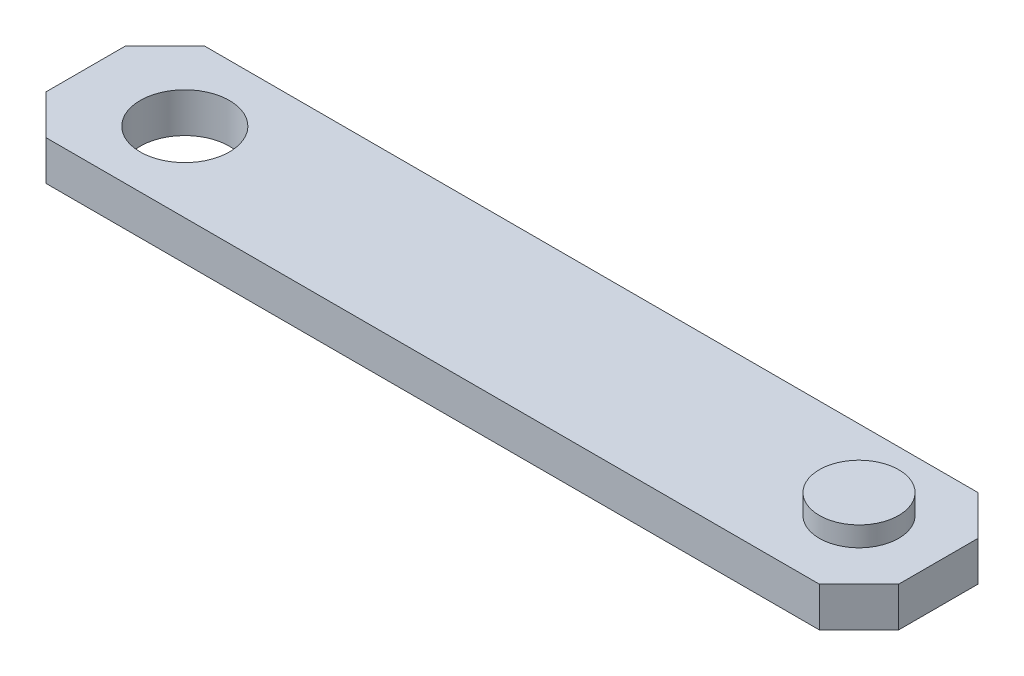
from build123d import *

# Parameters (mm, degrees)
SKETCH1_W           = 43
SKETCH1_H           = 8
BOSS_EXTRUDE1_DEPTH = 2
SKETCH2_R           = 2.25
CUT_EXTRUDE1_DEPTH  = 35.195745727
SKETCH3_R           = 2
BOSS_EXTRUDE2_DEPTH = 1
CHAMFER2_SIZE       = 2


with BuildPart() as part:
    # Sketch1 → Boss-Extrude1 (new body)
    with BuildSketch(Plane(origin=(0, 0, 0), x_dir=(1, 0, 0), z_dir=(0, 1, 0))):
        with Locations((11.806648575, 3.484396201)):
            Rectangle(SKETCH1_W, SKETCH1_H)
    extrude(amount=BOSS_EXTRUDE1_DEPTH)

    # Sketch2 → Cut-Extrude1 (cut, through all)
    with BuildSketch(Plane(origin=(0, 2, 0), x_dir=(1, 0, 0), z_dir=(0, 1, 0))):
        with Locations(Location((-4.693351425, 3.484396201, 0), (0, 0, 270))):
            Circle(SKETCH2_R)
    extrude(amount=-CUT_EXTRUDE1_DEPTH, mode=Mode.SUBTRACT)

    # Sketch3 → Boss-Extrude2 (add)
    with BuildSketch(Plane(origin=(0, 2, 0), x_dir=(1, 0, 0), z_dir=(0, 1, 0))):
        with Locations(Location((29.306648575, 3.484396201, 0), (0, 0, 270))):
            Circle(SKETCH3_R)
    extrude(amount=BOSS_EXTRUDE2_DEPTH)

    # Chamfer2
    chamfer2_edges = [part.edges().sort_by_distance(p)[0] for p in [
        (-9.693351425, 1, -7.484396201),
        (33.306648575, 1, -7.484396201),
        (33.306648575, 1, 0.515603799),
        (-9.693351425, 1, 0.515603799),
    ]]
    chamfer(chamfer2_edges, length=CHAMFER2_SIZE)


solid = part.part
